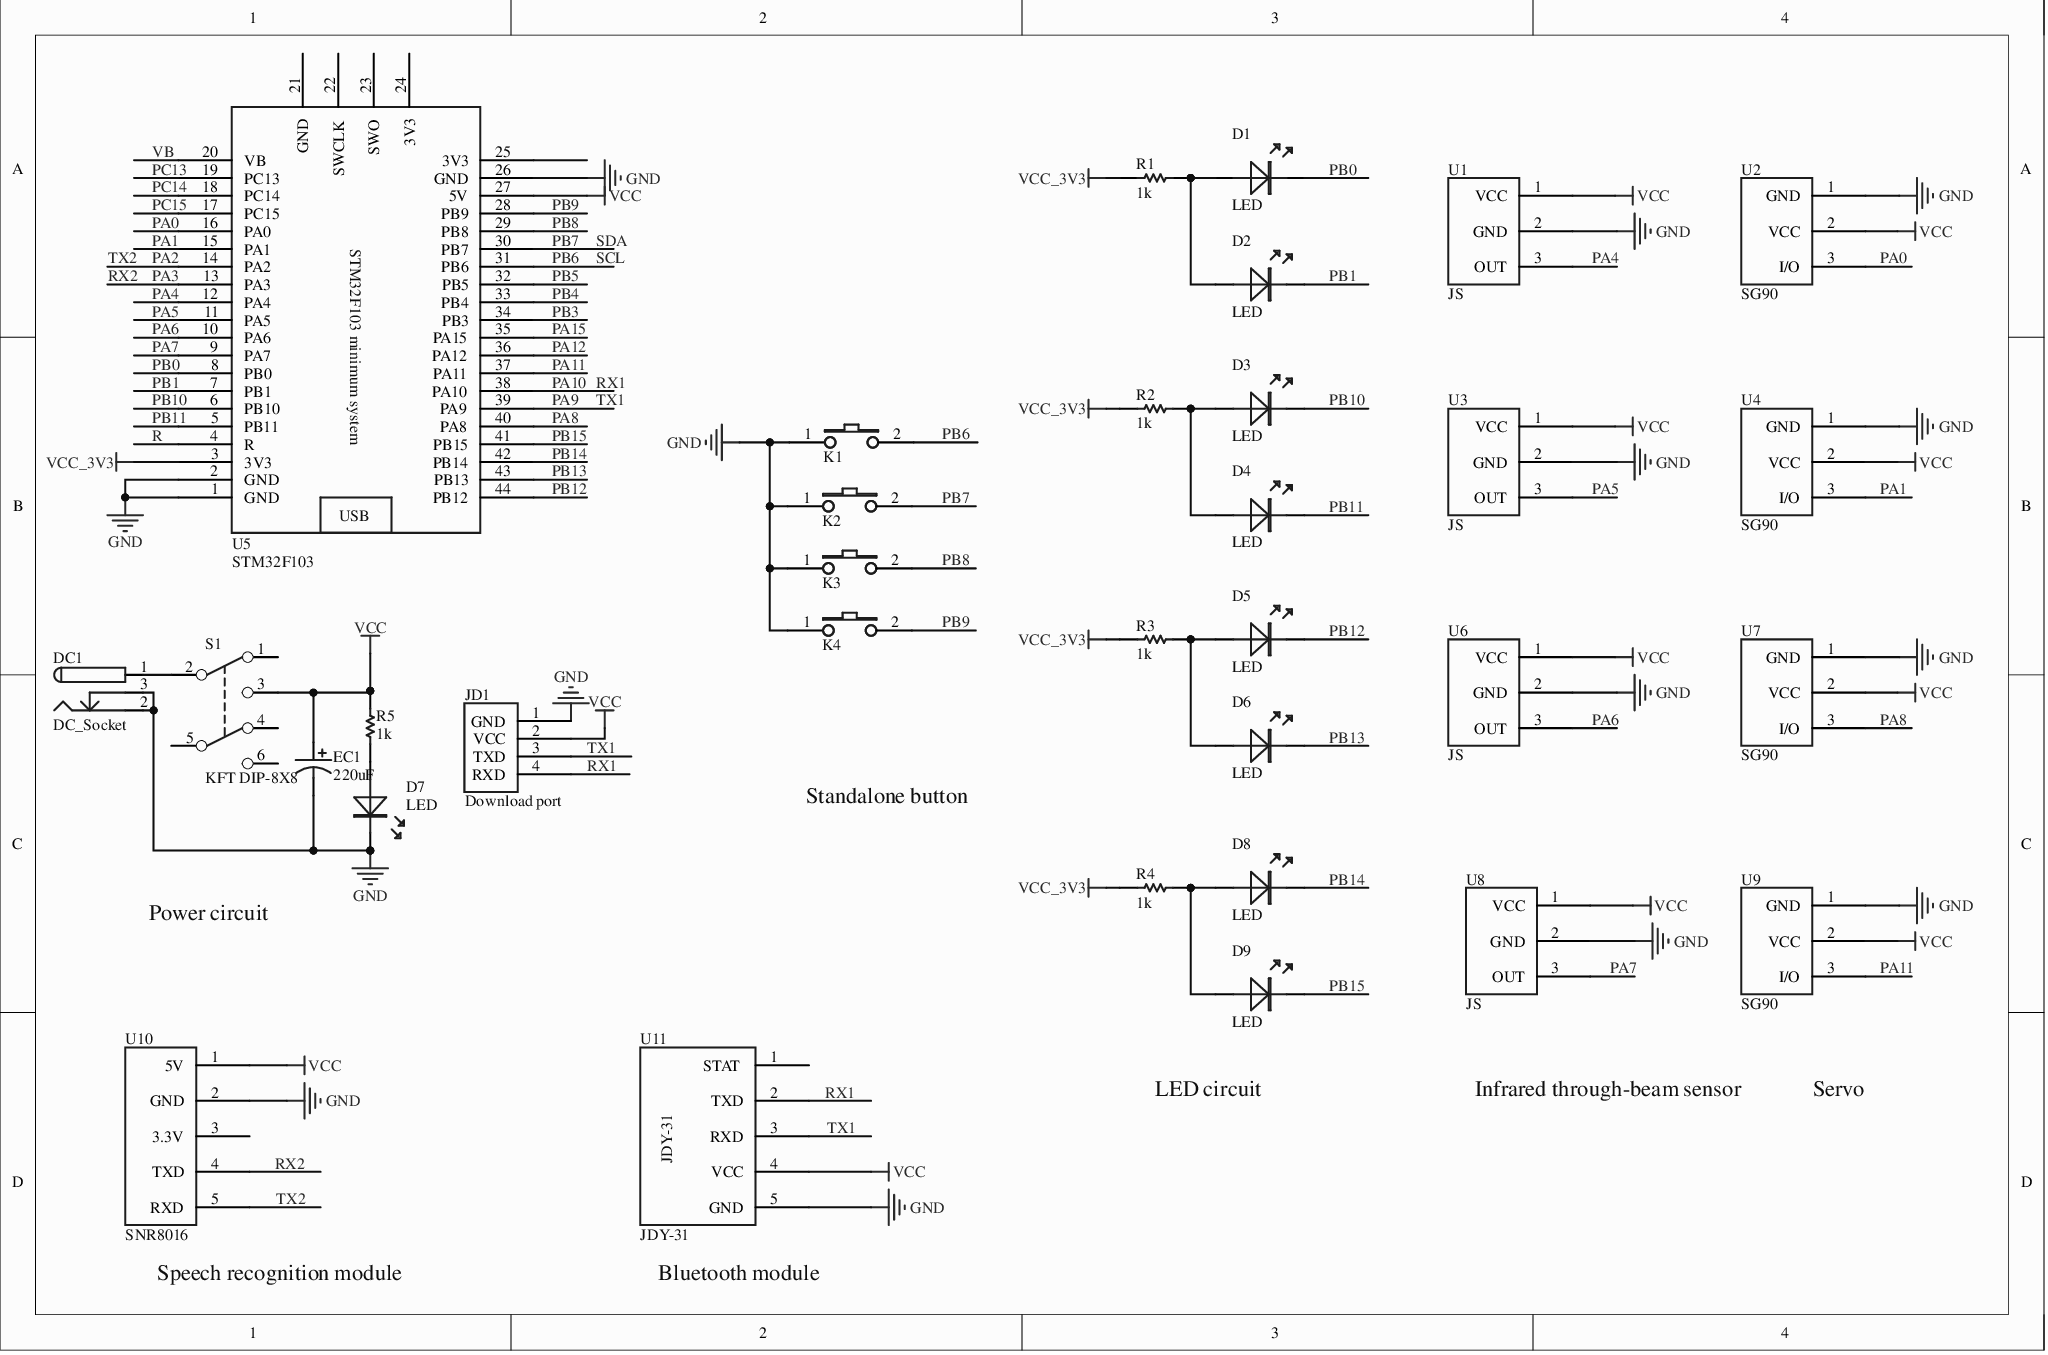
[diagram p0: MISC49886-2.schdoc]
# Altium project MISC49886.PrjPcb
1 sheet, 33 parts. Net scope: global (net labels, ports and power ports of the same name join across sheets).
Board file: MISC49886.pcbdoc

## Sheet MISC49886-2.schdoc
size 292 x 193 mm; Name: MISC49886

### Parts
D1  LED  [LED5-GRE]
D2  LED  [LED5-RED]
D3  LED  [LED5-GRE]
D4  LED  [LED5-RED]
D5  LED  [LED5-GRE]
D6  LED  [LED5-RED]
D7  LED  [LED5-GRE]
D8  LED  [LED5-GRE]
D9  LED  [LED5-RED]
DC1  DC_Socket  [DC-005]
EC1  220uF  [DIP-EC3.5X8X11.5]
JD1  Download port  [下载口]
K1  BUTTOM  [DIP-6X6X5]  (value not drawn)
K2  BUTTOM  [DIP-6X6X5]  (value not drawn)
K3  BUTTOM  [DIP-6X6X5]  (value not drawn)
K4  BUTTOM  [DIP-6X6X5]  (value not drawn)
R1  1k  [AXIAL0.3-1k]
R2  1k  [AXIAL0.3-1k]
R3  1k  [AXIAL0.3-1k]
R4  1k  [AXIAL0.3-1k]
R5  1k  [AXIAL0.3-1k]
S1  KFT DIP-8X8  [KFT DIP-8X8]
U1  JS  [JS]
U2  SG90  [SG90]
U3  JS  [JS]
U4  SG90  [SG90]
U5  STM32F103  [STM32F103]
U6  JS  [JS]
U7  SG90  [SG90]
U8  JS  [JS]
U9  SG90  [SG90]
U10  SNR8016  [SNR8016]
U11  JDY-31

### Nets
GND: D7.K DC1.2 DC1.3 EC1.2 JD1.1(GND) K1.1 K2.1 K3.1 K4.1 U1.2(GND) U2.1(GND) U3.2(GND) U4.1(GND) U5.1(GND) U5.2(GND) U5.26(GND) U6.2(GND) U7.1(GND) U8.2(GND) U9.1(GND) U10.2(GND) U11.5(GND)
VCC: EC1.1 JD1.2(VCC) R5.2 S1.3 U1.1(VCC) U2.2(VCC) U3.1(VCC) U4.2(VCC) U5.27(5V) U6.1(VCC) U7.2(VCC) U8.1(VCC) U9.2(VCC) U10.1(5V) U11.4(VCC)
VCC_3V3: R1.2 R2.2 R3.2 R4.2 U5.3(3V3)
PA0: U2.3(I/O) U5.16(PA0)
PA1: U4.3(I/O) U5.15(PA1)
PA2: U5.14(PA2) U10.5(RXD)  [also labelled TX2]
PA3: U5.13(PA3) U10.4(TXD)  [also labelled RX2]
PA4: U1.3(OUT) U5.12(PA4)
PA5: U3.3(OUT) U5.11(PA5)
PA6: U5.10(PA6) U6.3(OUT)
PA7: U5.9(PA7) U8.3(OUT)
PA8: U5.40(PA8) U7.3(I/O)
PA9: JD1.3(TXD) U5.39(PA9) U11.3(RXD)  [also labelled TX1]
PA10: JD1.4(RXD) U5.38(PA10) U11.2(TXD)  [also labelled RX1]
PA11: U5.37(PA11) U9.3(I/O)
PA12: U5.36(PA12)
PA15: U5.35(PA15)
PB0: D1.K U5.8(PB0)
PB1: D2.K U5.7(PB1)
PB3: U5.34(PB3)
PB4: U5.33(PB4)
PB5: U5.32(PB5)
PB6: K1.2 U5.31(PB6)  [also labelled SCL]
PB7: K2.2 U5.30(PB7)  [also labelled SDA]
PB8: K3.2 U5.29(PB8)
PB9: K4.2 U5.28(PB9)
PB10: D3.K U5.6(PB10)
PB11: D4.K U5.5(PB11)
PB12: D5.K U5.44(PB12)
PB13: D6.K U5.43(PB13)
PB14: D8.K U5.42(PB14)
PB15: D9.K U5.41(PB15)
PC13: U5.19(PC13)
PC14: U5.18(PC14)
PC15: U5.17(PC15)
R: U5.4(R)
VB: U5.20(VB)
NetD1_A: D1.A D2.A R1.1
NetD3_A: D3.A D4.A R2.1
NetD5_A: D5.A D6.A R3.1
NetD7_A: D7.A R5.1
NetD8_A: D8.A D9.A R4.1
NetDC1_1: DC1.1 S1.2

Not connected (* = marked no-connect by the designer): S1 1 4 5 6; U5 21(GND) 22(SWCLK) 23(SWO) 24(3V3) 25(3V3); U10 3(3.3V)*; U11 1(STAT)*

### Notes on the sheet
- Standalone button
- Power circuit
- LED circuit
- Infrared through-beam sensor
- Servo
- (near U10) Speech recognition module
- (near U11) Bluetooth module

### Library data of the parts
D1 = LED: Red LED; Origin Footprint: LED5-BLUE; OriginFootprint 3: LED5-YEL; UniqueId: 07a0d5848cd81316; AddInBom: yes; Device: LED; OriginFootprint 2: LED5-GRE; DesignItemID: LED; LibraryName: LED; SymbolName: LED; FootprintName: LED5-GRE
D2 = LED_1: Red LED; Origin Footprint: LED5-BLUE; OriginFootprint 2: LED5-GRE; OriginFootprint 3: LED5-YEL; UniqueId: fa5cd661465da5bc; AddInBom: yes; Device: LED_1; DesignItemID: LED; LibraryName: LED; SymbolName: LED; FootprintName: LED5-RED
D3 = LED: Red LED; Origin Footprint: LED5-BLUE; OriginFootprint 3: LED5-YEL; UniqueId: ce0e29427420bb9a; AddInBom: yes; Device: LED; OriginFootprint 2: LED5-GRE; DesignItemID: LED; LibraryName: LED; SymbolName: LED; FootprintName: LED5-GRE
D4 = LED_1: Red LED; Origin Footprint: LED5-BLUE; OriginFootprint 2: LED5-GRE; OriginFootprint 3: LED5-YEL; UniqueId: 671e3575a93d22ee; AddInBom: yes; Device: LED_1; DesignItemID: LED; LibraryName: LED; SymbolName: LED; FootprintName: LED5-RED
D5 = LED: Red LED; Origin Footprint: LED5-BLUE; OriginFootprint 3: LED5-YEL; UniqueId: f6a2299b727f22e5; AddInBom: yes; Device: LED; OriginFootprint 2: LED5-GRE; DesignItemID: LED; LibraryName: LED; SymbolName: LED; FootprintName: LED5-GRE
D6 = LED_1: Red LED; Origin Footprint: LED5-BLUE; OriginFootprint 2: LED5-GRE; OriginFootprint 3: LED5-YEL; UniqueId: da39aa9ccad1dedd; AddInBom: yes; Device: LED_1; DesignItemID: LED; LibraryName: LED; SymbolName: LED; FootprintName: LED5-RED
D7 = LED: Green LED; Origin Footprint: LED5-BLUE; OriginFootprint 2: LED5-RED; OriginFootprint 3: LED5-YEL; UniqueId: cc99b6ab75b61af5; AddInBom: yes; Device: LED; DesignItemID: LED; LibraryName: LED; SymbolName: LED; FootprintName: LED5-GRE
D8 = LED: Red LED; Origin Footprint: LED5-BLUE; OriginFootprint 3: LED5-YEL; UniqueId: fa1f7fcf59ad3572; AddInBom: yes; Device: LED; OriginFootprint 2: LED5-GRE; DesignItemID: LED; LibraryName: LED; SymbolName: LED; FootprintName: LED5-GRE
D9 = LED_1: Red LED; Origin Footprint: LED5-BLUE; OriginFootprint 2: LED5-GRE; OriginFootprint 3: LED5-YEL; UniqueId: 24b3e8ded7e5fe7b; AddInBom: yes; Device: LED_1; DesignItemID: LED; LibraryName: LED; SymbolName: LED; FootprintName: LED5-RED
DC1 = DC_Socket: Power socket; UniqueId: 918354ff671956d3; AddInBom: yes; ModelId: bc01fa3fdb994156aa7bd7788425d33b; Device: DC_Socket; DesignItemID: DC_Socket; LibraryName: Power socket; SymbolName: DC_Socket; FootprintName: DC-005; ModelName: DC-005
EC1 = 220uF: Through-hole electrolytic capacitor; UniqueId: 1f6a804da79fa676; SymbolName: DIP_ECAP; AddInBom: yes; Device: 220uF; DesignItemID: DIP_ECAP; LibraryName: Electrolytic capacitor--220uF; FootprintName: DIP-EC3.5X8X11.5
JD1 = 下载口_1: Device: Download port_1; UniqueId: 8d67e1bcb20313ce; AddInBom: yes; DesignItemID: 下载口; LibraryName: Download port; Description: Download port; SymbolName: Download port; FootprintName: Download port
K1 = BUTTOM: Button; UniqueId: 28855386baaab8ba; AddInBom: yes; Device: BUTTOM; DesignItemID: BUTTOM; LibraryName: Reference; SymbolName: BUTTOM; FootprintName: DIP-6X6X5
K2 = BUTTOM: Button; UniqueId: e2dee5ee6a5fdee0; AddInBom: yes; Device: BUTTOM; DesignItemID: BUTTOM; LibraryName: Reference; SymbolName: BUTTOM; FootprintName: DIP-6X6X5
K3 = BUTTOM: Button; UniqueId: 177bbada0502c5f7; AddInBom: yes; Device: BUTTOM; DesignItemID: BUTTOM; LibraryName: Reference; SymbolName: BUTTOM; FootprintName: DIP-6X6X5
K4 = BUTTOM: Button; UniqueId: 787baf109c0c5026; AddInBom: yes; Device: BUTTOM; DesignItemID: BUTTOM; LibraryName: Reference; SymbolName: BUTTOM; FootprintName: DIP-6X6X5
R1 = 1k: Resistor; Origin Footprint: AXIAL0.3-3.3k; OriginFootprint 2: AXIAL0.3-10k; UniqueId: 4e166b190d4de1c3; SymbolName: RES; AddInBom: yes; Device: 1k; DesignItemID: RES; LibraryName: Resistor; FootprintName: AXIAL0.3-1k
R2 = 1k: Resistor; Origin Footprint: AXIAL0.3-3.3k; OriginFootprint 2: AXIAL0.3-10k; UniqueId: 06442d24ab060343; SymbolName: RES; AddInBom: yes; Device: 1k; DesignItemID: RES; LibraryName: Resistor; FootprintName: AXIAL0.3-1k
R3 = 1k: Resistor; Origin Footprint: AXIAL0.3-3.3k; OriginFootprint 2: AXIAL0.3-10k; UniqueId: 6e26aea592918673; SymbolName: RES; AddInBom: yes; Device: 1k; DesignItemID: RES; LibraryName: Resistor; FootprintName: AXIAL0.3-1k
R4 = 1k: Resistor; Origin Footprint: AXIAL0.3-3.3k; OriginFootprint 2: AXIAL0.3-10k; UniqueId: 49359f7360e76581; SymbolName: RES; AddInBom: yes; Device: 1k; DesignItemID: RES; LibraryName: Resistor; FootprintName: AXIAL0.3-1k
R5 = 1k: Resistor; Origin Footprint: AXIAL0.3-3.3k; OriginFootprint 2: AXIAL0.3-10k; UniqueId: 96bd3269827a783e; SymbolName: RES; AddInBom: yes; Device: 1k; DesignItemID: RES; LibraryName: Resistor; FootprintName: AXIAL0.3-1k
S1 = KFT DIP-8X8_1: Self-locking button; UniqueId: da892dff24010eb4; AddInBom: yes; Device: KFT DIP-8X8_1; DesignItemID: KFT DIP-8X8; LibraryName: Self-locking button; SymbolName: KFT DIP-8X8; FootprintName: KFT DIP-8X8
U1 = JS_2: Infrared through-beam sensor--counting; UniqueId: 48a4a086d8c42a18; AddInBom: yes; Device: JS_2; DesignItemID: JS; LibraryName: Infrared through-beam sensor-counting; SymbolName: JS; FootprintName: JS
U2 = SG90_1: Servo; UniqueId: d74c11912b695046; AddInBom: yes; Device: SG90_1; DesignItemID: SG90; LibraryName: Servo; SymbolName: SG90; FootprintName: SG90
U3 = JS_2: Infrared through-beam sensor--counting; UniqueId: eac3f191c372887e; AddInBom: yes; Device: JS_2; DesignItemID: JS; LibraryName: Infrared through-beam sensor-counting; SymbolName: JS; FootprintName: JS
U4 = SG90_1: Servo; UniqueId: e5d1bee62801ccc5; AddInBom: yes; Device: SG90_1; DesignItemID: SG90; LibraryName: Servo; SymbolName: SG90; FootprintName: SG90
U5 = STM32F103_1: UniqueId: 65fd737caad1a168; AddInBom: yes; Device: STM32F103_1; DesignItemID: STM32F103; LibraryName: Custom schematic symbol library; Description: STM32F103; SymbolName: STM32F103; FootprintName: STM32F103
U6 = JS_2: Infrared through-beam sensor--counting; UniqueId: cb0a5e759a2bc85d; AddInBom: yes; Device: JS_2; DesignItemID: JS; LibraryName: Infrared through-beam sensor-counting; SymbolName: JS; FootprintName: JS
U7 = SG90_1: Servo; UniqueId: 917392894f3a2a5c; AddInBom: yes; Device: SG90_1; DesignItemID: SG90; LibraryName: Servo; SymbolName: SG90; FootprintName: SG90
U8 = JS_2: Infrared through-beam sensor--counting; UniqueId: 379bb34d70e5da90; AddInBom: yes; Device: JS_2; DesignItemID: JS; LibraryName: Infrared through-beam sensor-counting; SymbolName: JS; FootprintName: JS
U9 = SG90_1: Servo; UniqueId: 0cf0c6d72374702e; AddInBom: yes; Device: SG90_1; DesignItemID: SG90; LibraryName: Servo; SymbolName: SG90; FootprintName: SG90
U10 = SNR8016_1: Speech recognition module; UniqueId: 5152fb4fa8412479; AddInBom: yes; Device: SNR8016_1; DesignItemID: SNR8016; LibraryName: Speech recognition; SymbolName: SNR8016; FootprintName: SNR8016
U11 = JDY-31: Bluetooth; UniqueId: 8cd974130b34484c; AddInBom: yes; Device: JDY-31; Origin Footprint: JDY-31; DesignItemID: JDY-31; LibraryName: Bluetooth--JDY-31; SymbolName: JDY-31